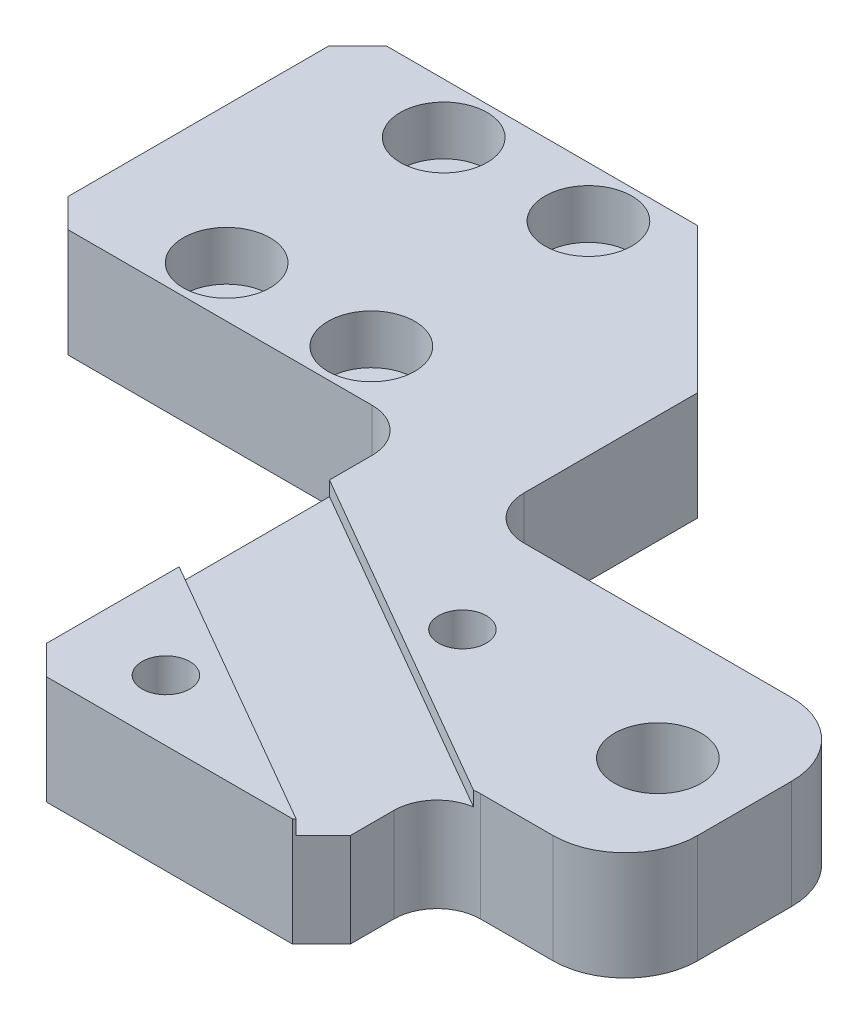
from build123d import *

# Parameters (mm, degrees)
SKETCH1_W                                          = 60
SKETCH1_H                                          = 49.5
BOSS_EXTRUDE1_DEPTH                                = 7.5
SKETCH2_W                                          = 26.5
SKETCH2_H                                          = 25
SKETCH2_W_2                                        = 13
SKETCH2_H_2                                        = 8
SKETCH2_W_3                                        = 26
SKETCH2_H_3                                        = 27.5
CUT_EXTRUDE1_DEPTH                                 = 40.60823778
HOLE_WIZARD_SOCKET_HEAD_CAP_SCREW_TYPE_D           = 3.4
HOLE_WIZARD_SOCKET_HEAD_CAP_SCREW_TYPE_CBORE_D     = 6
HOLE_WIZARD_SOCKET_HEAD_CAP_SCREW_TYPE_CBORE_DEPTH = 3.4
F_6_0_6_DIAMETER_HOLE1_D                           = 6
CUT_EXTRUDE2_DEPTH                                 = 1
FILLET1_R                                          = 5
CHAMFER1_SIZE                                      = 10
CHAMFER2_SIZE                                      = 2
FILLET2_R                                          = 3
M4_TAPPED_HOLE1_D                                  = 3.3
SKETCH10_R                                         = 2.75
CUT_EXTRUDE3_DEPTH                                 = 8


with BuildPart() as part:
    # Sketch1 → Boss-Extrude1 (new body)
    with BuildSketch(Plane(origin=(0, 0, 0), x_dir=(1, 0, 0), z_dir=(0, 1, 0))):
        Rectangle(SKETCH1_W, SKETCH1_H)
    extrude(amount=BOSS_EXTRUDE1_DEPTH)

    # Sketch2 → Cut-Extrude1 (cut, through all)
    with BuildSketch(Plane(origin=(0, 7.5, 0), x_dir=(1, 0, 0), z_dir=(0, 1, 0))):
        with Locations((16.75, 12.25)):
            Rectangle(SKETCH2_W, SKETCH2_H)
        with Locations((23.5, -20.75)):
            Rectangle(SKETCH2_W_2, SKETCH2_H_2)
        with Locations((-17, -11)):
            Rectangle(SKETCH2_W_3, SKETCH2_H_3)
    extrude(amount=-CUT_EXTRUDE1_DEPTH, mode=Mode.SUBTRACT)

    # Hole wizard: socket head cap screw, type 1 (through all)
    with Locations(Plane(origin=(0, 7.5, 0), x_dir=(1, 0, 0), z_dir=(0, 1, 0))):
        with Locations((-10.55, 21.25), (-20.55, 21.25), (-20.55, 6.25), (-10.55, 6.25)):
            CounterBoreHole(HOLE_WIZARD_SOCKET_HEAD_CAP_SCREW_TYPE_D / 2, HOLE_WIZARD_SOCKET_HEAD_CAP_SCREW_TYPE_CBORE_D / 2, HOLE_WIZARD_SOCKET_HEAD_CAP_SCREW_TYPE_CBORE_DEPTH)

    # Ø6.0 (6) Diameter Hole1 (through all)
    with Locations(Plane(origin=(0, 7.5, 0), x_dir=(1, 0, 0), z_dir=(0, 1, 0))):
        with Locations((24, -8.5)):
            Hole(F_6_0_6_DIAMETER_HOLE1_D / 2)

    # Sketch7 → Cut-Extrude2 (cut)
    with BuildSketch(Plane(origin=(0, 7.5, 0), x_dir=(1, 0, 0), z_dir=(0, 1, 0))):
        Polygon((-12.304041346, -8.790622211), (20.302775541, -27.616176718), (24.802775541, -19.821948084), (-7.804041346, -0.996393577), align=None)
    extrude(amount=-CUT_EXTRUDE2_DEPTH, mode=Mode.SUBTRACT)

    # Fillet1
    fillet1_edges = [part.edges().sort_by_distance(p)[0] for p in [
        (30, 3.75, 16.75),
        (30, 3.75, 0.25),
    ]]
    fillet(fillet1_edges, radius=FILLET1_R)

    # Chamfer1
    chamfer1_edges = [part.edges().sort_by_distance(p)[0] for p in [
        (3.5, 3.75, -24.75),
    ]]
    chamfer(chamfer1_edges, length=CHAMFER1_SIZE)

    # Chamfer2
    chamfer2_edges = [part.edges().sort_by_distance(p)[0] for p in [
        (17, 3.25, 24.75),
        (-4, 3.75, 24.75),
        (-30, 3.75, -2.75),
        (-30, 3.75, -24.75),
    ]]
    chamfer(chamfer2_edges, length=CHAMFER2_SIZE)

    # Fillet2
    fillet2_edges = [part.edges().sort_by_distance(p)[0] for p in [
        (3.5, 3.75, 0.25),
        (17, 3.25, 16.75),
        (-4, 3.75, -2.75),
    ]]
    fillet(fillet2_edges, radius=FILLET2_R)

    # M4 Tapped Hole1 (through all)
    with Locations(Plane(origin=(0, 7.5, 0), x_dir=(1, 0, 0), z_dir=(0, 1, 0))):
        with Locations((9.538573783, -7.545055475), (2.038573783, -20.535436532)):
            Hole(M4_TAPPED_HOLE1_D / 2)

    # Sketch10 → Cut-Extrude3 (cut)
    with BuildSketch(Plane.ZY.offset(30)):
        with Locations((-13.75, 3.75)):
            Circle(SKETCH10_R)
    extrude(amount=-CUT_EXTRUDE3_DEPTH, mode=Mode.SUBTRACT)


solid = part.part
